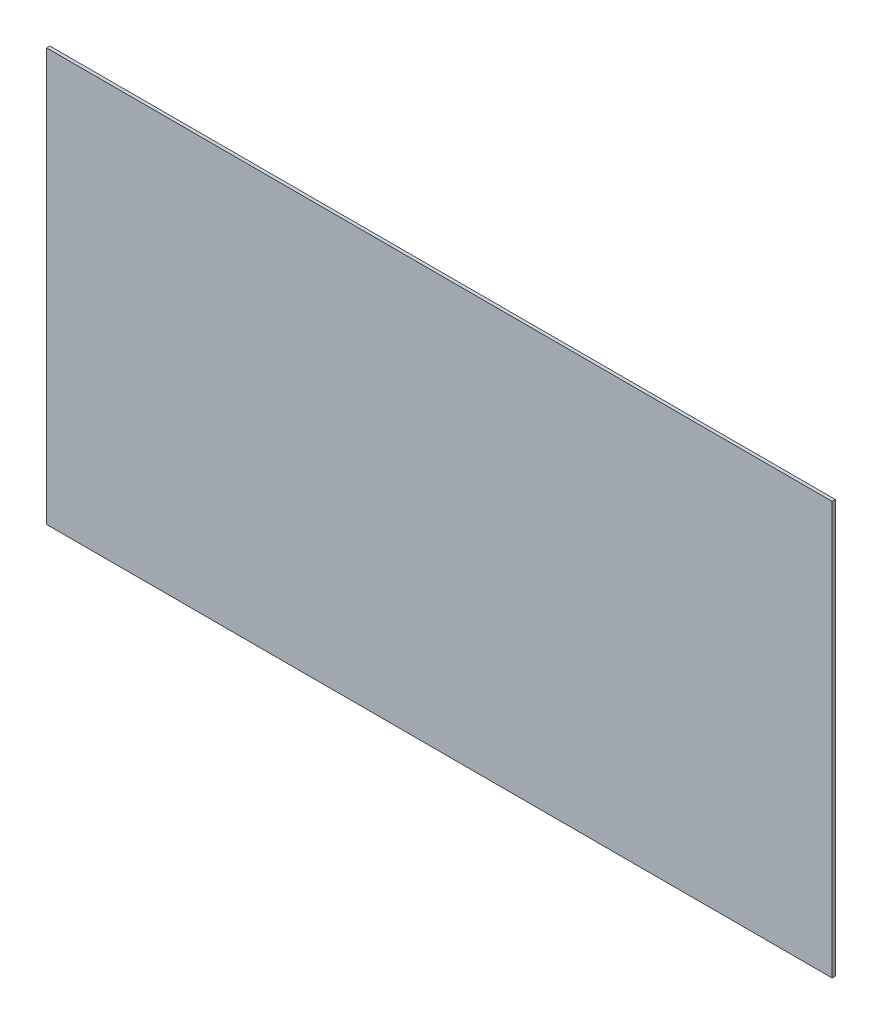
from build123d import *

# Parameters (mm, degrees)
SKETCH_1_W      = 1216
SKETCH_1_H      = 639
EXTRUDE_1_DEPTH = 5


with BuildPart() as part:
    # 草图1 → 凸台-拉伸1 (new body)
    with BuildSketch(Plane.XY):
        Rectangle(SKETCH_1_W, SKETCH_1_H)
    extrude(amount=EXTRUDE_1_DEPTH)


solid = part.part
